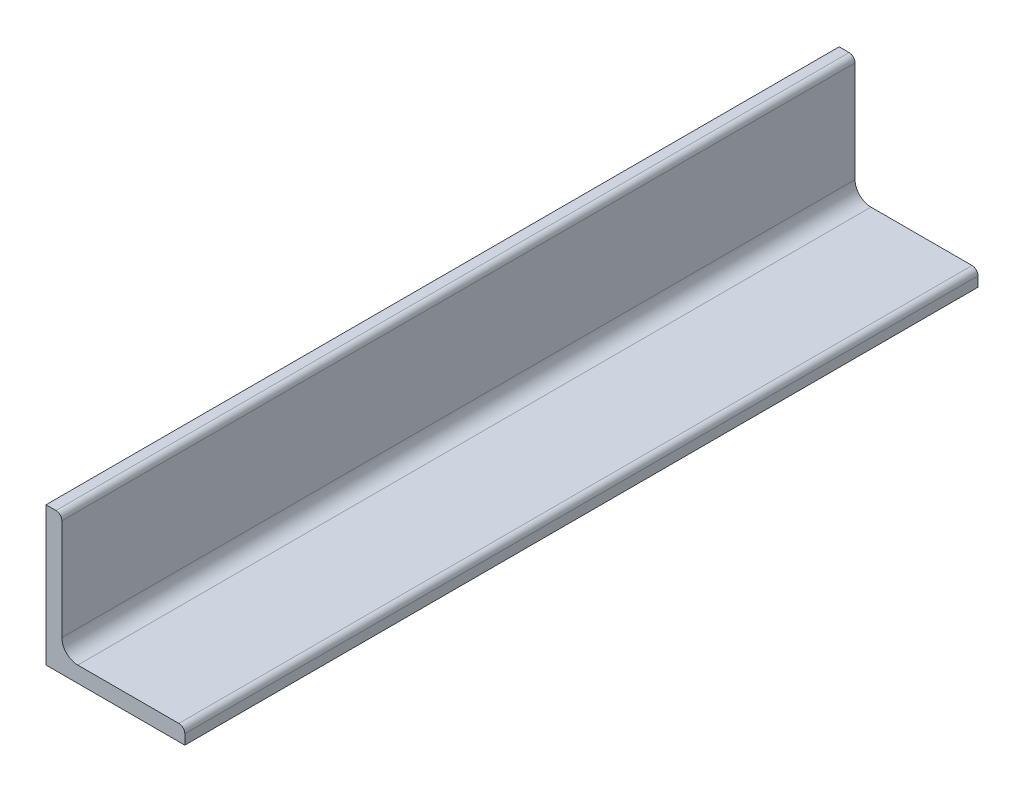
SolidWorks part; units mm, degrees
material "不锈钢角钢70×8/304"
ref_plane "Front Plane" through (0, 0, 0) normal (0, 0, 1) x (1, 0, 0)
ref_plane "Top Plane" through (0, 0, 0) normal (0, 1, 0) x (1, 0, 0)
ref_plane "Right Plane" through (0, 0, 0) normal (1, 0, 0) x (0, 0, -1)
sketch "Sketch1" plane through (0, 0, 0) normal (0, 0, 1) x (1, 0, 0)
  line L0 (0, 70) -> (0, 0)
  line L1 (0, 0) -> (70, 0)
  line L2 (70, 0) -> (70, 5)
  line L3 (67, 8) -> (16, 8)
  line L4 (8, 16) -> (8, 67)
  line L5 (5, 70) -> (0, 70)
  arc A0 (16, 8) -> (8, 16) centre (16, 16) cw
  arc A1 (70, 5) -> (67, 8) centre (67, 5) ccw
  arc A2 (8, 67) -> (5, 70) centre (5, 67) ccw
  dimension "D5" = 8
  dimension "D6" = 3
  dimension "D1" = 70
  dimension "D2" = 70
  dimension "D3" = 8
  dimension "D4" = 8
extrude "Boss-Extrude1" add sketch "Sketch1" along normal blind 400
ref_plane "Plane1" through (0, 0, 0) normal (0.7071, 0.7071, 0) x (0, 0, -1)
